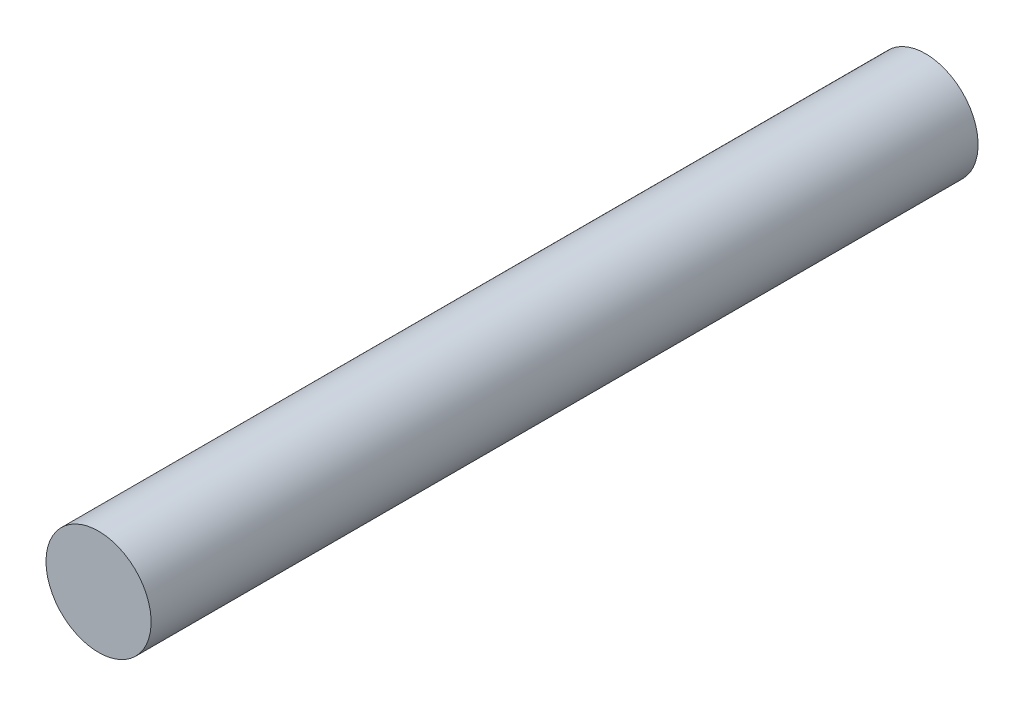
SolidWorks part; units mm, degrees
ref_plane "前视基准面" through (0, 0, 0) normal (0, 0, 1) x (1, 0, 0)
ref_plane "上视基准面" through (0, 0, 0) normal (0, 1, 0) x (1, 0, 0)
ref_plane "右视基准面" through (0, 0, 0) normal (1, 0, 0) x (0, 0, -1)
sketch "草图1" plane through (0, 0, 0) normal (0, 0, 1) x (1, 0, 0)
  circle A0 centre (0, 0) radius 15
  dimension "D1" = 30
extrude "凸台-拉伸1" add sketch "草图1" along normal blind 236
